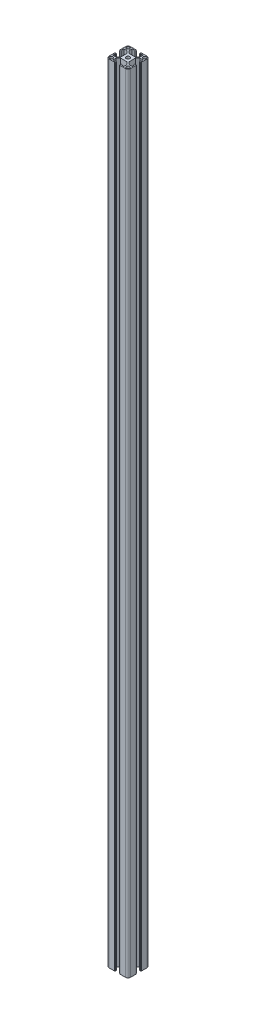
SolidWorks part; units mm, degrees
ref_plane "主视基准图" through (0, 0, 0) normal (0, 0, 1) x (1, 0, 0)
ref_plane "上视基准图" through (0, 0, 0) normal (0, 1, 0) x (1, 0, 0)
ref_plane "右视基准图" through (0, 0, 0) normal (1, 0, 0) x (0, 0, -1)
sketch "草图1" plane through (0, 0, 0) normal (0, 0, 1) x (1, 0, 0)
  line L0 (0, 0) -> (0, 1467)
  dimension "D1" = 1467
other "结构构件1"
ref_plane "基准面1" through (0, 0, 0) normal (0, 1, 0) x (-1, 0, 0)
sketch "Sketch16" plane through (0, 0, 0) normal (0, 1, 0) x (-1, 0, 0)
  line L0 (-5.1, 20) -> (-5.1, 19.5)
  line L1 (-5.1, 19.5) -> (-4.1, 19.5)
  line L2 (-4.1, 19.5) -> (-4.1, 17)
  line L3 (-6.1, 18) -> (-10.3, 18)
  line L4 (-15.5, -20) -> (-5.1, -20)
  line L5 (-20, -15.5) -> (-20, -5.1)
  line L6 (15.5, 20) -> (5.1, 20)
  line L7 (20, 15.5) -> (20, 5.1)
  line L8 (0, 14.8756) -> (0, 0) construction
  line L9 (0, 0) -> (14.1675, 0) construction
  line L10 (-10.3, 18) -> (-10.3, 12)
  line L11 (-10.3, 12) -> (-6, 7.7)
  line L12 (-6, 7.7) -> (6, 7.7)
  line L13 (10.3, 12) -> (6, 7.7)
  line L14 (10.3, 18) -> (10.3, 12)
  line L15 (6.1, 18) -> (10.3, 18)
  line L16 (4.1, 19.5) -> (4.1, 17)
  line L17 (5.1, 19.5) -> (4.1, 19.5)
  line L18 (5.1, 20) -> (5.1, 19.5)
  line L19 (-5.1, 20) -> (-15.5, 20)
  line L20 (20, 5.1) -> (19.5, 5.1)
  line L21 (0, 0) -> (-15.5563, 15.5563) construction
  line L22 (0, 0) -> (-15.5563, -15.5563) construction
  line L25 (19.5, 5.1) -> (19.5, 4.1)
  line L26 (19.5, 4.1) -> (17, 4.1)
  line L27 (17, 6.1) -> (17, 4.1)
  line L28 (18, 6.1) -> (17, 6.1)
  line L29 (18, 6.1) -> (18, 10.3)
  line L30 (18, 10.3) -> (12, 10.3)
  line L31 (12, 10.3) -> (7.7, 6)
  line L32 (7.7, 6) -> (7.7, -6)
  line L33 (12, -10.3) -> (7.7, -6)
  line L34 (18, -10.3) -> (12, -10.3)
  line L35 (18, -6.1) -> (18, -10.3)
  line L36 (18, -6.1) -> (17, -6.1)
  line L37 (17, -4.1) -> (17, -6.1)
  line L38 (19.5, -4.1) -> (17, -4.1)
  line L39 (19.5, -5.1) -> (19.5, -4.1)
  line L40 (20, -5.1) -> (19.5, -5.1)
  line L41 (5.1, -20) -> (5.1, -19.5)
  line L42 (5.1, -19.5) -> (4.1, -19.5)
  line L43 (4.1, -19.5) -> (4.1, -17)
  line L44 (6.1, -17) -> (4.1, -17)
  line L45 (6.1, -18) -> (6.1, -17)
  line L46 (6.1, -18) -> (10.3, -18)
  line L47 (10.3, -18) -> (10.3, -12)
  line L48 (10.3, -12) -> (6, -7.7)
  line L49 (6, -7.7) -> (-6, -7.7)
  line L50 (-10.3, -12) -> (-6, -7.7)
  line L51 (-10.3, -18) -> (-10.3, -12)
  line L52 (-6.1, -18) -> (-10.3, -18)
  line L53 (-6.1, -18) -> (-6.1, -17)
  line L54 (-4.1, -17) -> (-6.1, -17)
  line L55 (-4.1, -19.5) -> (-4.1, -17)
  line L56 (-5.1, -19.5) -> (-4.1, -19.5)
  line L57 (-5.1, -20) -> (-5.1, -19.5)
  line L58 (-20, -5.1) -> (-19.5, -5.1)
  line L59 (5.1, -20) -> (15.5, -20)
  line L60 (-20, 5.1) -> (-20, 15.5)
  line L61 (-19.5, -5.1) -> (-19.5, -4.1)
  line L62 (-6.1, 18) -> (-6.1, 17)
  line L63 (-6.1, 17) -> (-4.1, 17)
  line L64 (6.1, 18) -> (6.1, 17)
  line L65 (4.1, 17) -> (6.1, 17)
  line L66 (-19.5, -4.1) -> (-17, -4.1)
  line L71 (-17, -6.1) -> (-17, -4.1)
  line L72 (-18, -6.1) -> (-17, -6.1)
  line L73 (-18, -6.1) -> (-18, -10.3)
  line L74 (-18, -10.3) -> (-12, -10.3)
  line L75 (-12, -10.3) -> (-7.7, -6)
  line L76 (-7.7, -6) -> (-7.7, 6)
  line L77 (-12, 10.3) -> (-7.7, 6)
  line L78 (-18, 10.3) -> (-12, 10.3)
  line L79 (-18, 6.1) -> (-18, 10.3)
  line L80 (-18, 6.1) -> (-17, 6.1)
  line L81 (-17, 4.1) -> (-17, 6.1)
  line L82 (-19.5, 4.1) -> (-17, 4.1)
  line L83 (-19.5, 5.1) -> (-19.5, 4.1)
  line L84 (-20, 5.1) -> (-19.5, 5.1)
  line L85 (20, -5.1) -> (20, -15.5)
  circle A0 centre (0, 0) radius 3.4
  arc A1 (-20, 15.5) -> (-15.5, 20) centre (-15.5, 15.5) cw
  arc A2 (20, 15.5) -> (15.5, 20) centre (15.5, 15.5) ccw
  arc A3 (-15.5, -20) -> (-20, -15.5) centre (-15.5, -15.5) cw
  arc A4 (15.5, -20) -> (20, -15.5) centre (15.5, -15.5) ccw
  circle A5 centre (-15.5563, 15.5563) radius 3
  circle A6 centre (15.5563, 15.5563) radius 3
  circle A7 centre (15.5563, -15.5563) radius 3
  circle A8 centre (-15.5563, -15.5563) radius 3
  point P2 (0, 10)
  point P3 (0, 0)
  point P4 (0, 0)
  point P5 (-20, -20)
  point P6 (20, -20)
  point P7 (20, 20)
  point P8 (-20, 20)
  point P36 (-20, 20)
  point P39 (20, 20)
  dimension "D1" = 20.6
  dimension "D2" = 40
  dimension "D3" = 8.2
  dimension "D4" = 10.2
  dimension "D5" = 12.3
  dimension "D6" = 6.8
  dimension "D7" = 4.5
  dimension "D8" = 45
  dimension "D12" = 6
  dimension "D13" = 22
  dimension "D9" = 0.5
  dimension "D10" = 2
  dimension "D11" = 12
  dimension "D16" = 3
  dimension "D17" = 2
